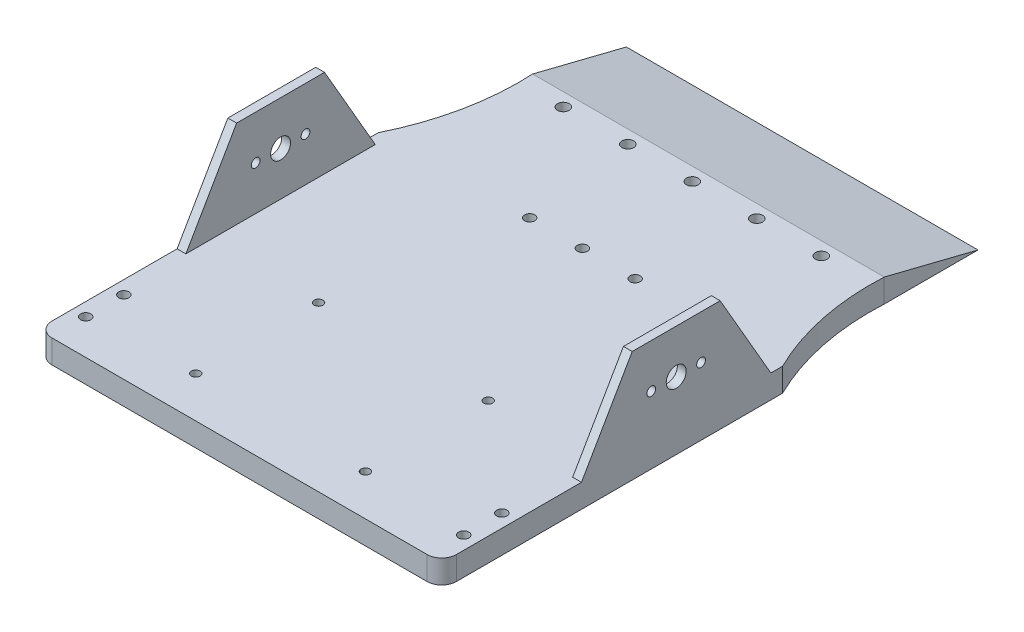
from build123d import *

# Parameters (mm, degrees)
SKETCH1_W                = 138
SKETCH1_H                = 160
BOSS_EXTRUDE1_DEPTH      = 8
SKETCH9_W                = 30
SKETCH9_H                = 38
SKETCH9_R                = 3.4
SKETCH9_R_2              = 1.5
BOSS_EXTRUDE4_DEPTH      = 3
RIB2_REACH               = 165.976
SKETCH10_WALL_W          = 364.592232036
SKETCH10_WALL_H          = 3
MIRROR4_COPY_1_REACH     = 165.976
MIRROR4_COPY_1_SKETCH_W  = 364.592232036
MIRROR4_COPY_1_SKETCH_H  = 3
CUT_EXTRUDE2_DEPTH       = 110.822584198
CUT_EXTRUDE2_DEPTH_BACK  = 110.822584198
SKETCH11_R               = 1.5
FILLET1_R                = 5
SKETCH12_R               = 1.75
CUT_EXTRUDE3_DEPTH       = 110.822584198
CUT_EXTRUDE4_DEPTH       = 110.822584198
BOSS_EXTRUDE5_DEPTH      = 60
BOSS_EXTRUDE5_DEPTH_BACK = 60
CUT_EXTRUDE5_DEPTH       = 137.926987844
CUT_EXTRUDE5_DEPTH_BACK  = 137.926987844
SKETCH15_R               = 2
SKETCH16_R               = 1.75
CUT_EXTRUDE6_DEPTH       = 50


with BuildPart() as part:
    # Sketch1 → Boss-Extrude1 (new body)
    with BuildSketch(Plane(origin=(0, 0, 0), x_dir=(1, 0, 0), z_dir=(0, 1, 0))):
        Rectangle(SKETCH1_W, SKETCH1_H)
    extrude(amount=BOSS_EXTRUDE1_DEPTH)

    # Sketch9 → Boss-Extrude4 (add)
    with BuildSketch(Plane.ZY.offset(69)):
        with Locations((0, 19)):
            Rectangle(SKETCH9_W, SKETCH9_H)
        with Locations((0, 23)):
            Circle(SKETCH9_R, mode=Mode.SUBTRACT)
        with Locations((8.5, 23)):
            Circle(SKETCH9_R_2, mode=Mode.SUBTRACT)
        with Locations((-8.5, 23)):
            Circle(SKETCH9_R_2, mode=Mode.SUBTRACT)
    boss_extrude4 = extrude(amount=-BOSS_EXTRUDE4_DEPTH)

    # Sketch10 wall → Rib2 (add, up to next)
    with BuildSketch(Plane(origin=(-69, 23, -23.660254038), x_dir=(0, -0.866025403781, -0.500000000007), z_dir=(0, -0.500000000007, 0.866025403781)), mode=Mode.PRIVATE) as rib2_sk1:
        with Locations((0, 1.5)):
            Rectangle(SKETCH10_WALL_W, SKETCH10_WALL_H)
    rib2_tool1 = extrude(rib2_sk1.sketch, amount=RIB2_REACH, mode=Mode.PRIVATE) - part.part
    rib2 = rib2_tool1.solids().sort_by_distance((-69, 23, -23.660254038))[0]
    add(rib2)

    # Mirror3: Rib2 across plane
    add(rib2.mirror(Plane.XY))

    # Mirror4: Boss-Extrude4, Rib2 across plane
    add(boss_extrude4.mirror(Plane(origin=(0, 0, 0), x_dir=(0, 0, 1), z_dir=(1, 0, 0))))
    add(rib2.mirror(Plane(origin=(0, 0, 0), x_dir=(0, 0, 1), z_dir=(1, 0, 0))))

    # Mirror4 copy 1 sketch → Mirror4 copy 1 (add, up to next)
    with BuildSketch(Plane(origin=(69, 23, 23.660254038), x_dir=(0, -0.866025403781, 0.500000000007), z_dir=(0, -0.500000000007, -0.866025403781)), mode=Mode.PRIVATE) as mirror4_copy_1_sk1:
        with Locations((0, 1.5)):
            Rectangle(MIRROR4_COPY_1_SKETCH_W, MIRROR4_COPY_1_SKETCH_H)
    mirror4_copy_1_tool1 = extrude(mirror4_copy_1_sk1.sketch, amount=MIRROR4_COPY_1_REACH, mode=Mode.PRIVATE) - part.part
    add(mirror4_copy_1_tool1.solids().sort_by_distance((69, 23, 23.660254038))[0])

    # Sketch11 → Cut-Extrude2 (cut, two sides: drawn at the far end of the back side and taken through both)
    with BuildSketch(Plane(origin=(0, 8, 0), x_dir=(1, 0, 0), z_dir=(0, 1, 0)).offset(-CUT_EXTRUDE2_DEPTH_BACK)):
        with Locations(Location((-28.95, -24.1, 0), (0, 0, 270))):
            Circle(SKETCH11_R)
        with Locations(Location((28.95, -24.1, 0), (0, 0, 90))):
            Circle(SKETCH11_R)
        with Locations(Location((-28.95, -66, 0), (0, 0, 90))):
            Circle(SKETCH11_R)
        with Locations(Location((28.95, -66, 0), (0, 0, 270))):
            Circle(SKETCH11_R)
    extrude(amount=CUT_EXTRUDE2_DEPTH + CUT_EXTRUDE2_DEPTH_BACK, mode=Mode.SUBTRACT)

    # Fillet1
    fillet1_edges = [part.edges().sort_by_distance(p)[0] for p in [
        (69, 4, 80),
        (-69, 4, 80),
        (-69, 4, -80),
        (69, 4, -80),
    ]]
    fillet(fillet1_edges, radius=FILLET1_R)

    # Sketch12 → Cut-Extrude3 (cut, symmetric)
    with BuildSketch(Plane(origin=(0, 8, 0), x_dir=(1, 0, 0), z_dir=(0, 1, 0))):
        with Locations(Location((64.5, -55, 0), (0, 0, 270))):
            Circle(SKETCH12_R)
        with Locations(Location((64.5, -68, 0), (0, 0, 270))):
            Circle(SKETCH12_R)
    cut_extrude3 = extrude(amount=CUT_EXTRUDE3_DEPTH, both=True, mode=Mode.SUBTRACT)

    # Mirror5: Cut-Extrude3 across plane
    add(cut_extrude3.mirror(Plane(origin=(0, 0, 0), x_dir=(0, 0, 1), z_dir=(1, 0, 0))), mode=Mode.SUBTRACT)

    # Sketch13 → Cut-Extrude4 (cut, symmetric)
    with BuildSketch(Plane(origin=(0, 8, 0), x_dir=(1, 0, 0), z_dir=(0, 1, 0))):
        with BuildLine():
            Line((60, 80), (80.385419548, 90.585690096))
            Line((80.385419548, 90.585690096), (122.100847158, 60.329129947))
            Line((122.100847158, 60.329129947), (69, 36.320508076))
            ThreePointArc((69, 36.320508076), (61.687085415, 57.580663247), (60, 80))
        make_face()
    cut_extrude4 = extrude(amount=CUT_EXTRUDE4_DEPTH, both=True, mode=Mode.SUBTRACT)

    # Mirror6: Cut-Extrude4 across plane
    add(cut_extrude4.mirror(Plane(origin=(0, 0, 0), x_dir=(0, 0, 1), z_dir=(1, 0, 0))), mode=Mode.SUBTRACT)

    # Sketch14 → Boss-Extrude5 (add, two sides: drawn at the far end of the back side and taken through both)
    with BuildSketch(Plane(origin=(0, 0, 0), x_dir=(0, 0, -1), z_dir=(1, 0, 0)).offset(-BOSS_EXTRUDE5_DEPTH_BACK)):
        Polygon((80, 0), (80, 8), (112, 0), align=None)
    extrude(amount=BOSS_EXTRUDE5_DEPTH + BOSS_EXTRUDE5_DEPTH_BACK)

    # Sketch15 → Cut-Extrude5 (cut, two sides: drawn at the far end of the back side and taken through both)
    with BuildSketch(Plane.XZ.offset(-CUT_EXTRUDE5_DEPTH_BACK)):
        with Locations(Location((-45, -75.5, 0), (0, 0, 270))):
            Circle(SKETCH15_R)
        with Locations(Location((-23, -75.5, 0), (0, 0, 270))):
            Circle(SKETCH15_R)
        with Locations(Location((-1, -75.5, 0), (0, 0, 270))):
            Circle(SKETCH15_R)
        with Locations(Location((21, -75.5, 0), (0, 0, 270))):
            Circle(SKETCH15_R)
        with Locations(Location((43, -75.5, 0), (0, 0, 270))):
            Circle(SKETCH15_R)
    extrude(amount=CUT_EXTRUDE5_DEPTH + CUT_EXTRUDE5_DEPTH_BACK, mode=Mode.SUBTRACT)

    # Sketch16 → Cut-Extrude6 (cut)
    with BuildSketch(Plane(origin=(0, 8, 0), x_dir=(1, 0, 0), z_dir=(0, 1, 0))):
        with Locations(Location((0, 37, 0), (0, 0, 270))):
            Circle(SKETCH16_R)
        with Locations(Location((18, 37, 0), (0, 0, 270))):
            Circle(SKETCH16_R)
        with Locations(Location((-18, 37, 0), (0, 0, 90))):
            Circle(SKETCH16_R)
    extrude(amount=-CUT_EXTRUDE6_DEPTH, mode=Mode.SUBTRACT)


solid = part.part
